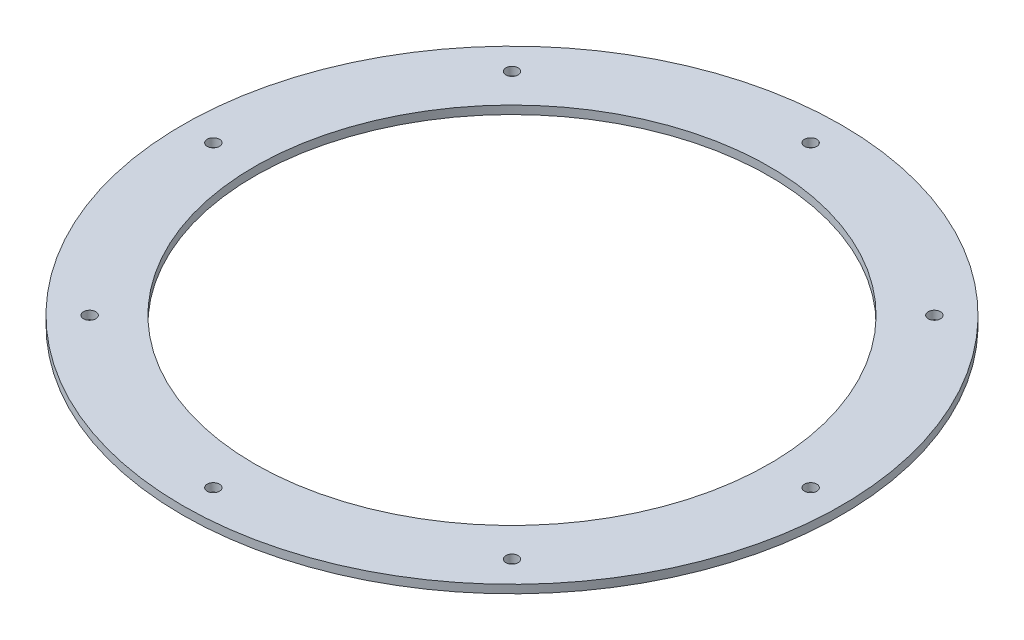
SolidWorks part; units mm, degrees
material "Q235"
ref_plane "前视基准面" through (0, 0, 0) normal (0, 0, 1) x (1, 0, 0)
ref_plane "上视基准面" through (0, 0, 0) normal (0, 1, 0) x (1, 0, 0)
ref_plane "右视基准面" through (0, 0, 0) normal (1, 0, 0) x (0, 0, -1)
sketch "草图1" plane through (0, 0, 0) normal (0, 1, 0) x (1, 0, 0)
  circle A0 centre (0, 0) radius 125
  circle A1 centre (0, 0) radius 160
  dimension "D1" = 250
  dimension "D2" = 320
extrude "凸台-拉伸1" add sketch "草图1" along normal blind 4
sketch "草图2" plane through (0, 4, 0) normal (0, 1, 0) x (1, 0, 0)
  circle A0 centre (0, 145) radius 3
  circle A1 centre (0, 0) radius 160 construction
  dimension "D1" = 6
  dimension "D2" = 145
extrude "切除-拉伸1" cut sketch "草图2" against normal through all
pattern_circular "阵列(圆周)1" count 8 over 360 about axis through (0, 0, 0) along (0, 1, 0) of "切除-拉伸1"
ref_plane "基准面1" through (-125, 0, 0) normal (1, 0, 0) x (0, 0, -1)
ref_plane "基准面2" through (0, 0, 125) normal (0, 0, 1) x (1, 0, 0)
ref_plane "基准面3" through (0, 0, -125) normal (0, 0, 1) x (1, 0, 0)
ref_plane "基准面4" through (125, 0, 0) normal (1, 0, 0) x (0, 0, -1)
